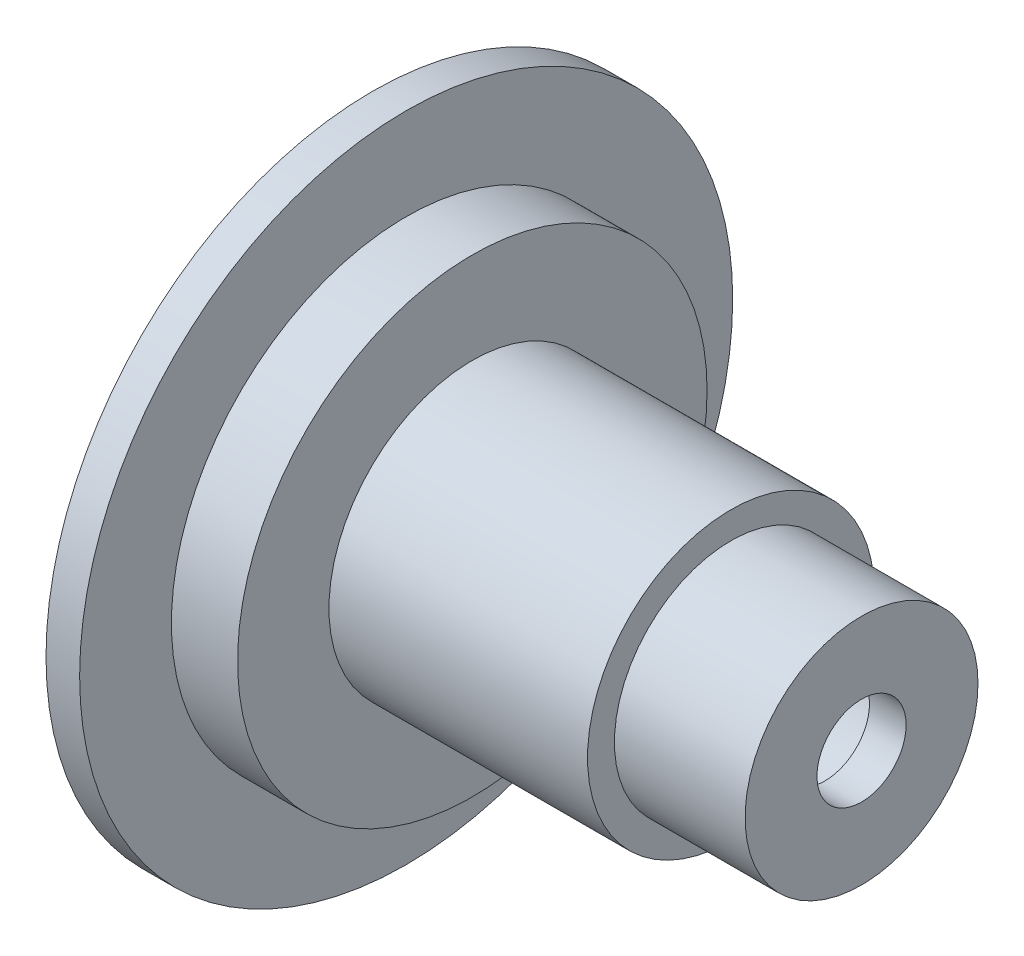
SolidWorks part; units mm, degrees
ref_plane "Front Plane" through (0, 0, 0) normal (0, 0, 1) x (1, 0, 0)
ref_plane "Top Plane" through (0, 0, 0) normal (0, 1, 0) x (1, 0, 0)
ref_plane "Right Plane" through (0, 0, 0) normal (1, 0, 0) x (0, 0, -1)
sketch "Sketch1" plane through (0, 0, 0) normal (0, 0, 1) x (1, 0, 0)
  line L0 (0, 0) -> (-11.7325, 0) construction
  line L1 (74.1426, 24.2791) -> (74.1426, 17.4546)
  line L2 (74.1426, 33.4546) -> (74.1426, -33.4546) construction
  line L3 (74.1426, 17.4546) -> (74.1426, -17.4546) construction
  line L4 (74.1426, 17.4546) -> (79.0608, 17.4546)
  line L5 (79.0608, 17.4546) -> (79.0608, 10.6596)
  line L6 (79.0608, 10.6596) -> (98.2863, 10.6596)
  line L7 (98.2863, -21.4326) -> (98.2863, 21.4326) construction
  line L8 (98.2863, 10.6596) -> (98.2863, 8.6596)
  line L9 (98.2863, 8.6596) -> (108, 8.6596)
  line L10 (108, -24.55) -> (108, 24.55) construction
  line L11 (71.6426, 24.2791) -> (71.6426, 14.9546)
  line L12 (71.6426, 14.9546) -> (76.5608, 14.9546)
  line L13 (76.5608, 14.9546) -> (76.5608, 8.1596)
  line L14 (76.5608, 8.1596) -> (95.7863, 8.1596)
  line L15 (95.7863, 8.1596) -> (95.7863, 6.1596)
  line L16 (95.7863, 6.1596) -> (105.2779, 6.1596)
  line L17 (108, 8.6596) -> (108, 3.3136)
  line L18 (108, 3.3136) -> (105.2779, 3.3136)
  line L19 (105.2779, 3.3136) -> (105.2779, 6.1596)
  line L20 (74.1426, 24.2791) -> (71.6426, 24.2791)
  line L21 (95.7863, 6.1596) -> (108, 6.1596) construction
  line L22 (108, 8.6596) -> (108, 3.3136)
  dimension "D1" = 2.5
revolve "Revolve1" add sketch "Sketch1" angle 360 about L0
